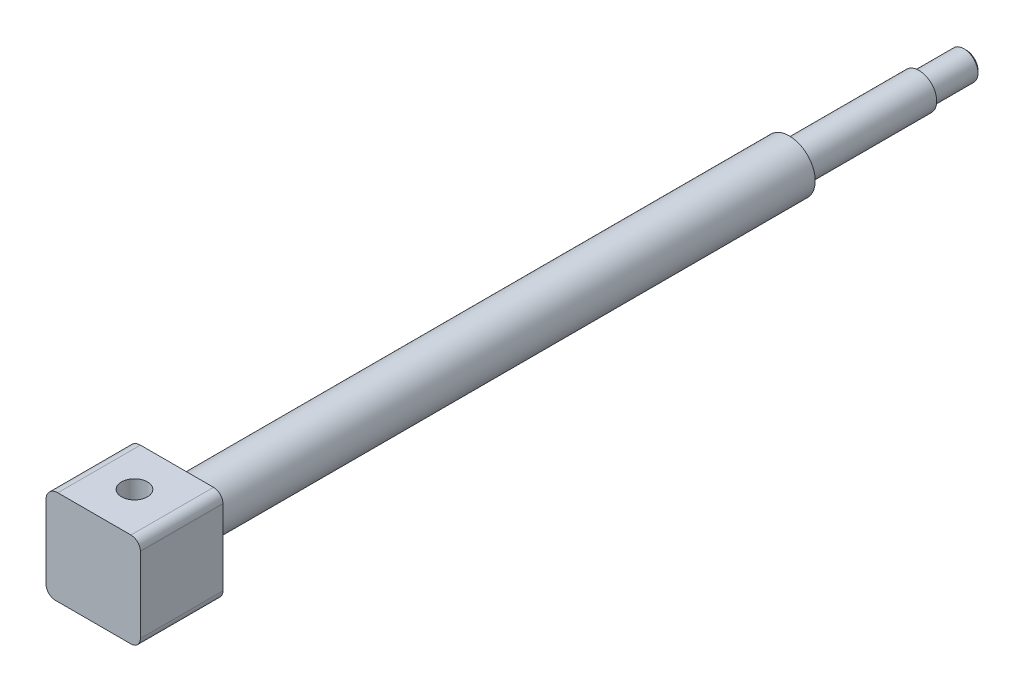
from build123d import *

# Parameters (mm, degrees)
BOSS_EXTRUDE2_DEPTH = 17.5
SKETCH3_R           = 5.5
CUT_EXTRUDE2_DEPTH  = 54
SKETCH4_R           = 11
BOSS_EXTRUDE3_DEPTH = 260
SKETCH5_R           = 7.5
BOSS_EXTRUDE4_DEPTH = 55
SKETCH6_R           = 6
BOSS_EXTRUDE5_DEPTH = 20
CHAMFER1_SIZE       = 1


with BuildPart() as part:
    # Sketch1 → Boss-Extrude2 (new, symmetric)
    with BuildSketch(Plane.XY):
        with BuildLine():
            Line((-15, 20), (16.011299973, 20))
            ThreePointArc((16.011299973, 20), (18.83173681, 18.83173681), (20, 16.011299973))
            Line((20, 16.011299973), (20, -16.011299973))
            ThreePointArc((20, -16.011299973), (18.83173681, -18.83173681), (16.011299973, -20))
            Line((16.011299973, -20), (-16.011299973, -20))
            ThreePointArc((-16.011299973, -20), (-18.83173681, -18.83173681), (-20, -16.011299973))
            Line((-20, -16.011299973), (-20, 15))
            ThreePointArc((-20, 15), (-18.535533906, 18.535533906), (-15, 20))
        make_face()
    extrude(amount=BOSS_EXTRUDE2_DEPTH, both=True)

    # Sketch3 → Cut-Extrude2 (cut)
    with BuildSketch(Plane(origin=(0, 20, 0), x_dir=(1, 0, 0), z_dir=(0, 1, 0))):
        with Locations(Location((0, 0, 0), (0, 0, 270))):
            Circle(SKETCH3_R)
    extrude(amount=-CUT_EXTRUDE2_DEPTH, mode=Mode.SUBTRACT)

    # Sketch4 → Boss-Extrude3 (add)
    with BuildSketch(Plane(origin=(0, 0, -17.5), x_dir=(-1, 0, 0), z_dir=(0, 0, -1))):
        Circle(SKETCH4_R)
    extrude(amount=BOSS_EXTRUDE3_DEPTH)

    # Sketch5 → Boss-Extrude4 (add)
    with BuildSketch(Plane(origin=(0, 0, -277.5), x_dir=(-1, 0, 0), z_dir=(0, 0, -1))):
        Circle(SKETCH5_R)
    extrude(amount=BOSS_EXTRUDE4_DEPTH)

    # Sketch6 → Boss-Extrude5 (add)
    with BuildSketch(Plane(origin=(0, 0, -332.5), x_dir=(-1, 0, 0), z_dir=(0, 0, -1))):
        Circle(SKETCH6_R)
    extrude(amount=BOSS_EXTRUDE5_DEPTH)

    # Chamfer1
    chamfer1_edges = [part.edges().sort_by_distance(p)[0] for p in [
        (6, 0, -352.5),
    ]]
    chamfer(chamfer1_edges, length=CHAMFER1_SIZE)


solid = part.part
